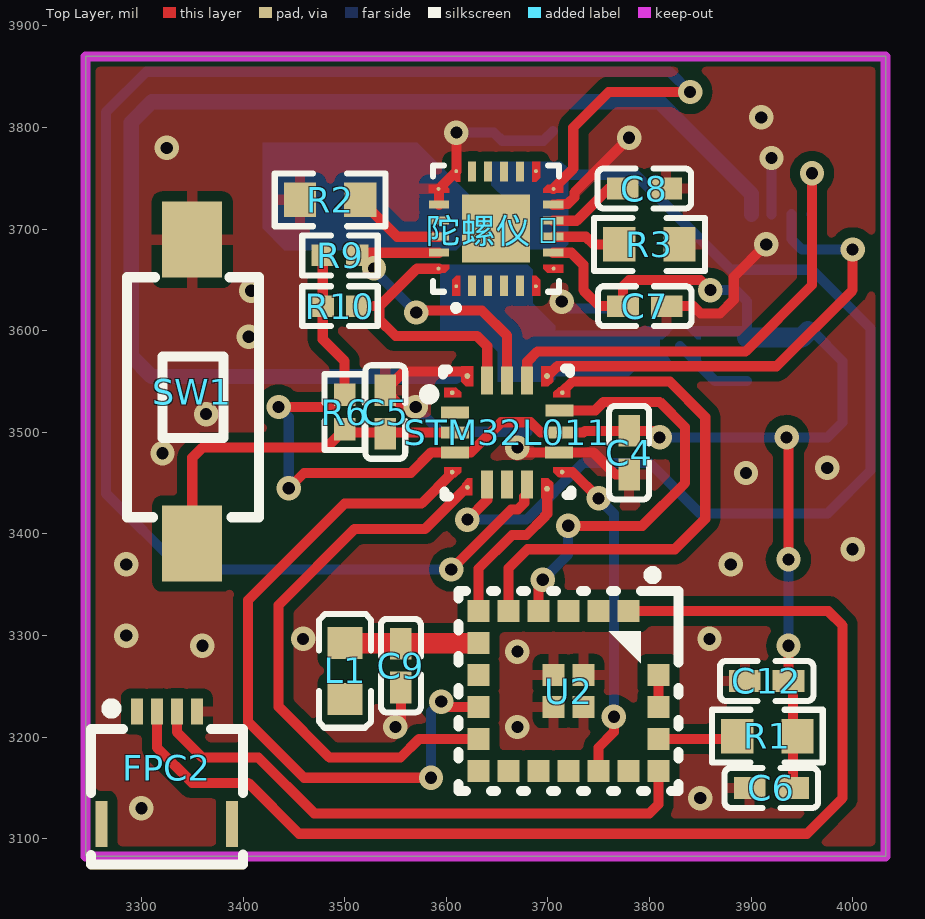
[diagram p0: Top Layer view]
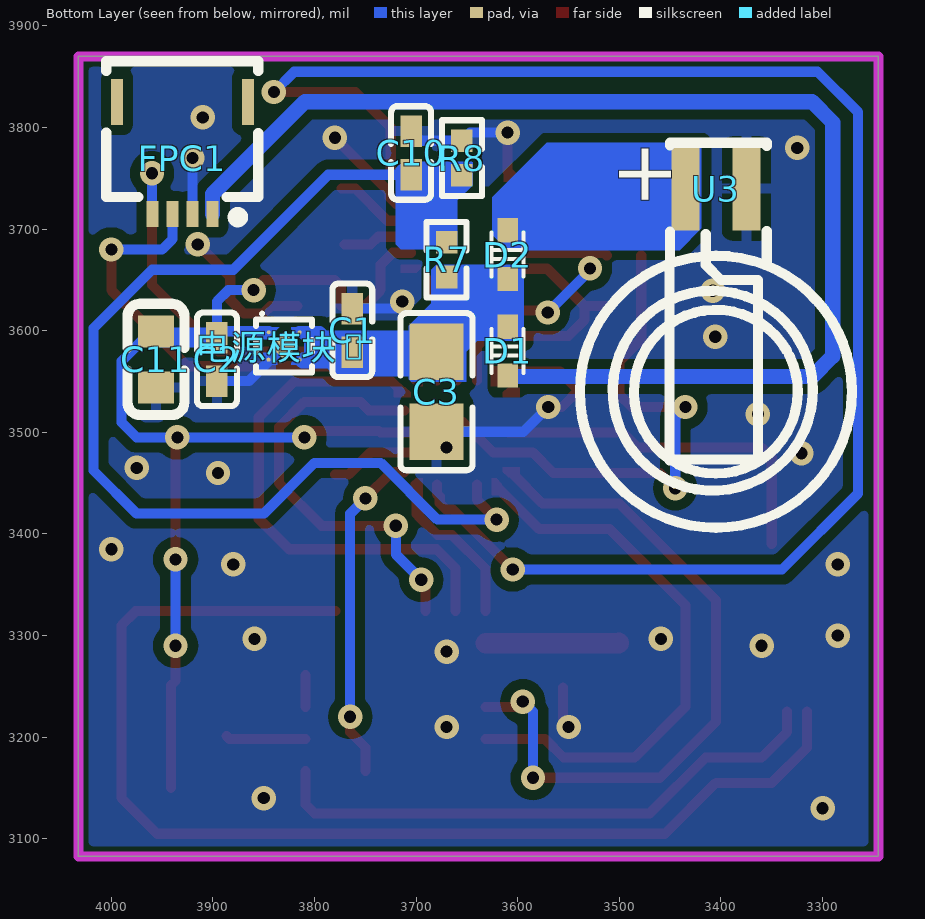
[diagram p1: Bottom Layer view, seen from below]
# Altium PCB MISC50958.pcbdoc
Units mil, origin at the board's own origin, x right, y up, seen from the top; angles counter-clockwise.
Board outline 787.4 x 787.4 mil, 2 copper layers (Top Layer, Bottom Layer), stack 62.206 mil thick; 31 components, 27 nets, 136 pads, 47 vias.

## Layer stack, top to bottom
Top Solder Mask Layer: solder mask 0.394, Dk 3.3
Top Layer: signal copper 1.379
Dielectric1: surface 59.449, FR4, Dk 4.5
Bottom Layer: signal copper 1.378
Bottom Solder Mask Layer: solder mask 0.394, Dk 3.3

## Board outline
3245,3870 3245,3082.6 4032.4,3082.6 4032.4,3870

## Design rules (kind name [scope] priority, off if disabled: settings)
BoardOutlineClearance copperThickness2oz_1 [All] p2 off: genericclearance=7.99 ignorepadtopadclearanceinfootprint=FALSE except(0: Arc-SplitContinuation Track-SplitContinuation SMDPad-SplitContinuation THPad-SplitContinuation Via-SplitContinuation Fill-SplitContinuation Region-SplitContinuation Poly-SplitContinuation Text-SplitContinuation Hole-SplitContinuation; 5.98: Arc-OutlineEdge Track-OutlineEdge SMDPad-OutlineEdge THPad-OutlineEdge Via-OutlineEdge Fill-OutlineEdge Region-OutlineEdge Text-OutlineEdge Hole-OutlineEdge SMDPad-CutoutEdge THPad-CutoutEdge Via-CutoutEdge Fill-CutoutEdge Region-CutoutEdge Text-CutoutEdge Hole-CutoutEdge; 10: Poly-OutlineEdge Poly-CutoutEdge; 11.81: Arc-CutoutEdge Track-CutoutEdge)
BoardOutlineClearance Plane_innerPlane_1 [All] p4 off: genericclearance=4.02 ignorepadtopadclearanceinfootprint=FALSE except(0: Arc-SplitContinuation Track-SplitContinuation SMDPad-SplitContinuation THPad-SplitContinuation Via-SplitContinuation Fill-SplitContinuation Region-SplitContinuation Poly-SplitContinuation Text-SplitContinuation Hole-SplitContinuation; 5.98: Arc-OutlineEdge Track-OutlineEdge SMDPad-OutlineEdge THPad-OutlineEdge Via-OutlineEdge Fill-OutlineEdge Region-OutlineEdge Text-OutlineEdge Hole-OutlineEdge SMDPad-CutoutEdge THPad-CutoutEdge Via-CutoutEdge Fill-CutoutEdge Region-CutoutEdge Text-CutoutEdge Hole-CutoutEdge; 10: Poly-OutlineEdge Poly-CutoutEdge; 11.81: Arc-CutoutEdge Track-CutoutEdge)
BoardOutlineClearance Copper_copperRegion_1 [All] p6 off: genericclearance=4.02 ignorepadtopadclearanceinfootprint=FALSE except(0: Arc-SplitContinuation Track-SplitContinuation SMDPad-SplitContinuation THPad-SplitContinuation Via-SplitContinuation Fill-SplitContinuation Region-SplitContinuation Poly-SplitContinuation Text-SplitContinuation Hole-SplitContinuation; 5.98: Arc-OutlineEdge Track-OutlineEdge SMDPad-OutlineEdge THPad-OutlineEdge Via-OutlineEdge Fill-OutlineEdge Region-OutlineEdge Text-OutlineEdge Hole-OutlineEdge SMDPad-CutoutEdge THPad-CutoutEdge Via-CutoutEdge Fill-CutoutEdge Region-CutoutEdge Text-CutoutEdge Hole-CutoutEdge; 10: Poly-OutlineEdge Poly-CutoutEdge; 11.81: Arc-CutoutEdge Track-CutoutEdge)
BoardOutlineClearance copperThickness1oz_1 [All] p8: genericclearance=4.02 ignorepadtopadclearanceinfootprint=FALSE except(0: Arc-SplitContinuation Track-SplitContinuation SMDPad-SplitContinuation THPad-SplitContinuation Via-SplitContinuation Fill-SplitContinuation Region-SplitContinuation Poly-SplitContinuation Text-SplitContinuation Hole-SplitContinuation; 5.98: Arc-OutlineEdge Track-OutlineEdge SMDPad-OutlineEdge THPad-OutlineEdge Via-OutlineEdge Fill-OutlineEdge Region-OutlineEdge Text-OutlineEdge Hole-OutlineEdge SMDPad-CutoutEdge THPad-CutoutEdge Via-CutoutEdge Fill-CutoutEdge Region-CutoutEdge Text-CutoutEdge Hole-CutoutEdge; 10: Poly-OutlineEdge Poly-CutoutEdge; 11.81: Arc-CutoutEdge Track-CutoutEdge)
Clearance copperThickness2oz [All] p1 off: gap=7.99 ignorepadtopadclearanceinfootprint=FALSE except(5.98: SMDPad-Track SMDPad-SMDPad THPad-Track SMDPad-THPad THPad-THPad Track-Via SMDPad-Via THPad-Via Via-Via Fill-Track Region-Track Fill-SMDPad Region-SMDPad Fill-THPad Region-THPad Fill-Via Region-Via Fill-Fill Fill-Region Region-Region Arc-Track Arc-SMDPad Arc-THPad Arc-Via Fill-Arc Region-Arc Arc-Arc Text-Track SMDPad-Text Text-THPad Text-Via Fill-Text Region-Text Arc-Text Text-Text Hole-Track Hole-SMDPad Hole-THPad Hole-Via Fill-Hole Region-Hole Hole-Arc Hole-Text; 10: Poly-Track Poly-SMDPad Poly-THPad Poly-Via Poly-Fill Poly-Region Poly-Poly Poly-Arc Poly-Text Poly-Hole)
Clearance Plane_innerPlane [All] p3 off: gap=4.02 ignorepadtopadclearanceinfootprint=FALSE except(5.98: SMDPad-Track SMDPad-SMDPad THPad-Track SMDPad-THPad THPad-THPad Track-Via SMDPad-Via THPad-Via Via-Via Fill-Track Region-Track Fill-SMDPad Region-SMDPad Fill-THPad Region-THPad Fill-Via Region-Via Fill-Fill Fill-Region Region-Region Arc-Track Arc-SMDPad Arc-THPad Arc-Via Fill-Arc Region-Arc Arc-Arc Text-Track SMDPad-Text Text-THPad Text-Via Fill-Text Region-Text Arc-Text Text-Text Hole-Track Hole-SMDPad Hole-THPad Hole-Via Fill-Hole Region-Hole Hole-Arc Hole-Text; 10: Poly-Track Poly-SMDPad Poly-THPad Poly-Via Poly-Fill Poly-Region Poly-Poly Poly-Arc Poly-Text Poly-Hole)
Clearance Copper_copperRegion [All] p5 off: gap=4.02 ignorepadtopadclearanceinfootprint=FALSE except(5.98: SMDPad-Track SMDPad-SMDPad THPad-Track SMDPad-THPad THPad-THPad Track-Via SMDPad-Via THPad-Via Via-Via Fill-Track Region-Track Fill-SMDPad Region-SMDPad Fill-THPad Region-THPad Fill-Via Region-Via Fill-Fill Fill-Region Region-Region Arc-Track Arc-SMDPad Arc-THPad Arc-Via Fill-Arc Region-Arc Arc-Arc Text-Track SMDPad-Text Text-THPad Text-Via Fill-Text Region-Text Arc-Text Text-Text Hole-Track Hole-SMDPad Hole-THPad Hole-Via Fill-Hole Region-Hole Hole-Arc Hole-Text; 10: Poly-Track Poly-SMDPad Poly-THPad Poly-Via Poly-Fill Poly-Region Poly-Poly Poly-Arc Poly-Text Poly-Hole)
Clearance copperThickness1oz [All] p7: gap=4.02 ignorepadtopadclearanceinfootprint=FALSE except(5.98: SMDPad-Track SMDPad-SMDPad THPad-Track SMDPad-THPad THPad-THPad Track-Via SMDPad-Via THPad-Via Via-Via Fill-Track Region-Track Fill-SMDPad Region-SMDPad Fill-THPad Region-THPad Fill-Via Region-Via Fill-Fill Fill-Region Region-Region Arc-Track Arc-SMDPad Arc-THPad Arc-Via Fill-Arc Region-Arc Arc-Arc Text-Track SMDPad-Text Text-THPad Text-Via Fill-Text Region-Text Arc-Text Text-Text Hole-Track Hole-SMDPad Hole-THPad Hole-Via Fill-Hole Region-Hole Hole-Arc Hole-Text; 10: Poly-Track Poly-SMDPad Poly-THPad Poly-Via Poly-Fill Poly-Region Poly-Poly Poly-Arc Poly-Text Poly-Hole)
DiffPairsRouting differentialPair [All] p1: maxlimit=6 minlimit=6 mostfreqgap=6 toplayer_minwidth=5 toplayer_prefwidth=10 toplayer_maxwidth=100 toplayer_mingap=6 toplayer_prefgap=6 toplayer_maxgap=6 bottomlayer_minwidth=5 bottomlayer_prefwidth=10 bottomlayer_maxwidth=100 bottomlayer_mingap=6 bottomlayer_prefgap=6 bottomlayer_maxgap=6 maxuncoupledlength=10
HoleToHoleClearance otherClearance [All] p1: gap=11.8 allowstackedmicrovias=TRUE
Length netLength [All] p1: minlimit=0 maxlimit=0
PasteMaskExpansion pasteMaskExpansion [All] p1: expansion=0
PlaneConnect innerPlane [All] p1: planeconnectstyle=Relief reliefexpansion=20 reliefentries=4 reliefconductorwidth=10 reliefairgap=10
PolygonConnect copperRegion [(InNet('GND'))] p1: connectstyle=Relief reliefconductorwidth=10 reliefentries=4 polygonreliefangle="90 Angle" airgapwidth=10 via.connectstyle=Relief via.reliefconductorwidth=10 via.reliefentries=4 via.polygonreliefangle="90 Angle" via.airgapwidth=10
RoutingVias viaSize [All] p1: holewidth=12.01 width=24.02 viastyle="Through Hole" minholewidth=11.81 minwidth=19.68 maxholewidth=248.03 maxwidth=393.7
SolderMaskExpansion solderMaskExpansion [IsVia] p1: expansion=-1000 istentingtop=TRUE
SolderMaskExpansion solderMaskExpansion [All] p2: expansion=2 istentingtop=FALSE
Width copperThickness2oz_2 [All] p1 off: maxlimit=100 minlimit=8 preferedwidth=10
Width copperThickness1oz_2 [All] p2: maxlimit=100 minlimit=5 preferedwidth=10

## Components (designator, comment, footprint, x,y, rotation, side; value= is the part's Value field where it differs from the comment)
C1 "1uF" C0402 3762.88,3600.39 r270 bottom
C2 "1uF" C0402 3896.09,3571.84 r90 bottom
C3 "10uF" C0805 3680,3540 r90 bottom
C4 "1uF" C0402 3780,3480 r90 top
C5 "100nF" C0402 3540,3520 r270 top
C6 "100nF" C0402 3920,3150 r0 top
C7 "100nF" C0402 3795.44,3624.22 r180 top
C8 "100nF" C0402 3795,3740 r0 top
C9 "100nF" C0402 3555.37,3270.32 r90 top
C10 "1uF" C0402 3705,3775 r270 bottom
C11 "100nF" C0603 3956.09,3571.84 r90 bottom
C12 "100nF" C0402 3915.37,3255.32 r0 top
D1 "1N4148G" SOD-723_L1.0-W0.6-P1.4-RD 3610,3580 r270 bottom
D2 "1N4148G" SOD-723_L1.0-W0.6-P1.4-RD 3610,3675 r90 bottom
FPC1 "HC-FPC-05-10-4RLTAG" FPC-SMD_4P-P0.50_HCTL_HC-FPC-05-10-4RLTAG 3930,3770 r180 bottom
FPC2 "HC-FPC-05-10-4RLTAG" FPC-SMD_4P-P0.50_HCTL_HC-FPC-05-10-4RLTAG 3325,3170 r180 top
L1 "10uH" L0603 3500.37,3265.32 r90 top
R1 "10K" R0603 3916.06,3201 r0 top
R2 "10K" R0603 3485.78,3728.88 r0 top
R3 "10K" R0603 3800,3685 r180 top
R6 "10kΩ" R0402 3500,3520 r270 top
R7 "20kΩ" R0402 3670,3670 r270 bottom
R8 "10kΩ" R0402 3655,3770 r270 bottom
R9 "4.7kΩ" R0402 3495.44,3674.22 r0 top
R10 "4.7kΩ" R0402 3495.44,3624.22 r0 top
STM32L011 "STM32L011F4U6TR" QFN-20_L3.0-W3.0-P0.50-BL 3660,3500 r180 top
SW1 "TS-1101-C-W" SW-SMD_L6.0-W3.3-LS8.0 3350,3540 r90 top
U2 "HJ-185IMH" LGA-24_L5.5-W5.0-P0.75-BL-EP 3720.37,3245.32 r180 top
U3 "MS621FE-FL11E" BAT-SMD_FL11E 3405,3740 r90 bottom
电源模块1 "1.8V转压" ZQFN-4L_L1.0-W1.0-P0.63-BL-EP 3830,3585 r270 bottom
陀螺仪1 "ICM-20948" QFN-24_L3.0-W3.0-P0.40-BL-EP 3649.05,3700.44 r0 top

## Footprints (in the part's own frame and the unit in brackets; to place one, negate y for a bottom-side part, rotate by r counter-clockwise, add the part's x,y. Pads: shape width x height; smd on the part's side, far side on the other; paste and mask are expansions set on the pad)
BAT-SMD_FL11E [mm]
  rect 2.1x0.7 smd paste+0 mask+0.05: 1(0,0.762) 2(0,-0.762)
  silkscreen extent -8.48,-3.4 1.14,3.4
C0402 [mm]
  rect 0.79x0.54 smd paste-100 mask+0.051: 1(-0.545,0) 2(0.545,0)
  silkscreen extent -1.17,-0.5 1.17,0.5
C0603 [mm]
  rect 0.8x0.9 smd: 1(-0.7,0) 2(0.7,0)
  silkscreen extent -1.39,-0.71 1.39,0.71
C0805 [mm]
  rect 1.41x1.35 smd paste-100 mask+0.051: 1(-1,0) 2(1,0)
  silkscreen extent -1.96,-0.9 1.96,0.9
FPC-SMD_4P-P0.50_HCTL_HC-FPC-05-10-4RLTAG [mm]
  rect 0.3x0.65 smd paste+0 mask+0.05: 1(0.75,-1.405) 2(0.25,-1.405) 3(-0.25,-1.405) 4(-0.75,-1.405)
  rect 0.3x1.15 smd paste+0 mask+0.05: 5(-1.635,1.405) 6(1.635,1.405)
  silkscreen extent -1.9,-1.6 1.89,2.42
L0603 [mm]
  rect 0.8x0.864 smd paste-100 mask+0.051: 1(-0.7,0) 2(0.7,0)
  silkscreen extent -1.42,-0.65 1.42,0.65
LGA-24_L5.5-W5.0-P0.75-BL-EP [mm]
  rect 0.55x0.55 smd paste+0 mask+0.05: 1(-1.5,-2) 2(-0.75,-2) 3(0,-2) 4(0.75,-2) 5(1.5,-2) 6(2.25,-2) 7(2.25,-1.2) 8(2.25,-0.4) 9(2.25,0.4) 10(2.25,1.2) 11(2.25,2) 12(1.5,2) 13(0.75,2) 14(0,2) 15(-0.75,2) 16(-1.5,2) 17(-2.25,2) 18(-2.25,1.2) 19(-2.25,0.4) 20(-2.25,-0.4) 21(-0.375,0.4) 22(0.375,0.4) 23(0.375,-0.4) 24(-0.375,-0.4)
  silkscreen extent -2.75,-3 2.75,2.5
QFN-20_L3.0-W3.0-P0.50-BL [mm]
  round 0.117 smd: 1(1.378,-0.99) 5(1.377,0.993) 6(0.994,1.377) 11(-1.373,0.992) 15(-1.378,-0.993)
  rect 0.7x0.3 smd paste+0 mask+0.05: 2(1.301,-0.5) 3(1.301,0) 4(1.301,0.5) 12(-1.299,0.5) 13(-1.299,0) 14(-1.312,-0.55)
  rect 0.3x0.7 smd paste+0 mask+0.05: 7(0.501,1.3) 8(0.001,1.3) 9(-0.499,1.3) 17(-0.499,-1.3) 18(0.001,-1.3) 19(0.501,-1.3)
  round 0.145 smd: 10(-0.994,1.41) 16(-0.994,-1.41) 20(0.996,-1.41)
  Top Layer region: 1.151,-1.65 0.851,-1.65 0.851,-1.15 1.031,-1.15 1.151,-1.26
  Top Layer region: -1.149,-1.65 -0.849,-1.65 -0.849,-1.15 -1.029,-1.15 -1.149,-1.26
  Top Layer region: -1.149,1.65 -0.849,1.65 -0.849,1.15 -1.029,1.15 -1.149,1.26
  Top Layer region: 1.574,1.124 1.574,0.878 1.497,0.876 1.15,0.876 1.15,0.999 1.289,1.125
  Top Layer region: 1.125,1.574 0.878,1.574 0.877,1.496 0.877,1.149 1,1.149 1.126,1.288
  Top Layer region: -1.575,-1.125 -1.575,-0.877 -1.151,-0.877 -1.151,-1 -1.29,-1.126
  Top Layer region: -1.571,1.123 -1.571,0.876 -1.493,0.875 -1.146,0.875 -1.146,0.998 -1.285,1.124
  Top Layer region: 1.575,-1.121 1.575,-0.875 1.498,-0.873 1.151,-0.873 1.151,-0.997 1.29,-1.123
  silkscreen extent -1.6,-1.6 2.08,1.6
QFN-24_L3.0-W3.0-P0.40-BL-EP [mm]
  round 0.097 smd: 1(-0.996,-1.439) 6(0.997,-1.439) 7(1.439,-0.997) 12(1.439,0.996) 13(0.997,1.439) 18(-0.997,1.439) 19(-1.439,0.997) 24(-1.439,-0.997)
  rect 0.2x0.505 smd paste-100 mask+0.051: 2(-0.6,-1.427) 3(-0.2,-1.427) 4(0.2,-1.427) 5(0.6,-1.427) 14(0.6,1.427) 15(0.2,1.427) 16(-0.2,1.427) 17(-0.6,1.427)
  rect 0.505x0.2 smd paste-100 mask+0.051: 8(1.427,-0.6) 9(1.427,-0.2) 10(1.427,0.2) 11(1.427,0.6) 20(-1.427,0.6) 21(-1.427,0.2) 22(-1.427,-0.2) 23(-1.427,-0.6)
  rect 1.7x1.7 smd paste-100 mask+0.051: 25(0,0)
  Top Layer region: -1.1,1.68 -0.9,1.68 -0.9,1.175 -1,1.174 -1.1,1.274
  Top Layer region: -1.68,-1.1 -1.274,-1.1 -1.174,-1 -1.175,-0.9 -1.68,-0.9
  Top Layer region: 1.68,-1.1 1.275,-1.1 1.175,-1 1.175,-0.9 1.68,-0.9
  Top Layer region: 1.68,1.1 1.274,1.1 1.174,1 1.175,0.9 1.68,0.9
  Top Layer region: 1.1,1.68 0.9,1.68 0.9,1.175 1,1.174 1.1,1.274
  Top Layer region: -1.1,-1.68 -0.9,-1.68 -0.9,-1.175 -1,-1.174 -1.1,-1.275
  Top Layer region: 1.1,-1.68 0.9,-1.68 0.9,-1.175 1,-1.175 1.1,-1.275
  Top Layer region: -1.68,1.1 -1.274,1.1 -1.174,1 -1.175,0.9 -1.68,0.9
  silkscreen extent -1.58,-2.05 1.58,1.58
R0402 [mm]
  rect 0.566x0.54 smd paste-100 mask+0.051: 1(-0.433,0) 2(0.433,0)
  silkscreen extent -0.94,-0.5 0.94,0.5
R0603 [mil]
  rect 31.75x34.02 smd paste-3937.01 mask+2: 1(-29.66,0) 2(29.66,0)
  silkscreen extent -55,-26 55,26
SOD-723_L1.0-W0.6-P1.4-RD [mil]
  rect 24x20 smd: 1(-24.05,0) 2(24.05,0)
  silkscreen extent -22,-16 22,16
SW-SMD_L6.0-W3.3-LS8.0 [mm]
  rect 1.9x1.5 smd: 1(-3.8,0) 2(3.8,0)
  silkscreen extent -3.14,-1.67 2.86,1.63
ZQFN-4L_L1.0-W1.0-P0.63-BL-EP [mm]
  round 0.099 smd: 1(-0.343,-0.385)
  round 0.101 smd: 2(0.341,-0.389)
  round 0.1 smd: 3(0.341,0.389) 4(-0.341,0.389)
  rect 0.5x0.5 smd rot 45: 5(0,0)
  Top Layer region: -0.163,-0.525 -0.463,-0.525 -0.463,-0.125 -0.163,-0.425
  Top Layer region: 0.163,0.525 0.463,0.525 0.463,0.175 0.413,0.175 0.163,0.425
  Top Layer region: -0.463,0.175 -0.463,0.525 -0.163,0.525 -0.163,0.475 -0.163,0.425 -0.413,0.175
  Top Layer region: 0.463,-0.175 0.463,-0.525 0.163,-0.525 0.163,-0.425 0.413,-0.175
  silkscreen extent -0.83,-0.7 0.66,0.7

## Via types
v1: diameter 24.02, hole 12, Top Layer to Bottom Layer, 47 vias

## Nets (pads, with @x,y where several pads share a name; then routed paths per layer and width w, separated by ;. In a path a pad name is that pad's centre, name@x,y a point inside that pad or via, vN(x,y) a via of type N, cw(c..) or ccw(c..) an arc to the next point about the centre after c; other vN are vias at no path point)
3.3V: D1.2 FPC1.1 | length 1235.2
  Bottom Layer w15: D1.2 3609.05,3555 3310,3555 3290,3575 3290,3805 3310.5,3825.5 3809.5,3825.5 3900.47,3734.53 FPC1.1
$1N2563: C8.1 陀螺仪1.10 | length 81.4
  Top Layer w10: 陀螺仪1.10 3728.31,3708.31 3760,3740 C8.1
$1N2566: U2.19 U2.20 | length 31.5
  Top Layer w10: U2.19 U2.20
$1N3256: R1.1 U2.18 | length 78.7
  Top Layer w10: U2.18 3883.47,3198.07 R1.1
$1N3260: R2.2 陀螺仪1.22 | length 92.4
  Top Layer w10: R2.2 3551.75,3692.57 陀螺仪1.22
$1N3265: C9.2 L1.2 U2.7 | length 131.6
  Top Layer w20: L1.2 3500.68,3292.55 U2.7
$1N3266: R3.2 陀螺仪1.9 | length 68.2
  Top Layer w10: 陀螺仪1.9 3737.43,3692.57 3745,3685 R3.2
$1N3268: D2.2 U3.1
BATADC: C10.2 R7.1 R8.2 STM32L011.7 | length 1015.9
  Top Layer w10: v1(3620.86,3414.14) 3640.29,3433.56 STM32L011.7
  Bottom Layer w10: v1(3620.86,3414.14) 3679.14,3414.14 3735,3470 3800,3470 3850,3420 3975,3420 4017.5,3462.5 4017.5,3602.5 3960,3660 3880,3660 3786.46,3753.54 C10.2
BLE_CLK: FPC2.2 U2.1 | length 1146.4
  Top Layer w10: FPC2.2 3315.16,3189.84 3350,3155 3405,3155 3455,3105 3955,3105 3990,3140 3990,3310 3975.95,3324.05 U2.1
BLE_SWD: FPC2.3 U2.17 | length 563.8
  Top Layer w10: FPC2.3 3334.84,3205.16 3360,3180 3415,3180 3470,3125 3800,3125 3808.95,3133.95 U2.17
BLUE-RESET: STM32L011.8
BLUE_RX: STM32L011.15 U2.5 | length 516.3
  Top Layer w10: U2.5 3661.31,3366.31 3680,3385 3825,3385 3855,3415 3855,3515 3820,3550 3724.26,3550 STM32L011.15@3713.67,3539.41
BLUE_TX: STM32L011.14 U2.4 | length 420.6
  Top Layer w10: U2.4 3690.84,3350.84 v1(3695,3355) ; STM32L011.14 3746.66,3521.66 3755,3530 3810,3530 3835,3505 3835,3450 3792.99,3407.99 v1(3720,3407.99)
  Bottom Layer w10: v1(3695,3355) 3720,3380 v1(3720,3407.99)
GND: C1.1 C2.1 C3.1 C4.1 C5.1 C6.1 C7.1 C8.2 C9.1 C10.1 C11.1 C12.1 FPC1.2 FPC2.4 R2.1 R3.1 R8.1 STM32L011.12 STM32L011.20 SW1.2 U2.21 U2.22 U2.23 U2.24 U3.2 电源模块1.2 电源模块1.5 陀螺仪1.11 陀螺仪1.18 陀螺仪1.19 陀螺仪1.20 | length 1030.5
  Top Layer w10: v1(3550,3210) 3555.37,3215.37 C9.1 ; v1(3570,3525) 3556.46,3525 C5.1 3558.54,3560 3615.72,3560 STM32L011.20@3620.61,3555.12 ; 陀螺仪1.20 3592.85,3739.81 3609.68,3756.64 3610,3756.96 v1(3610,3795) ; v1(3670,3485) 3674.68,3480.32 STM32L011.12 3744.68,3480.32 3766.46,3458.54 C4.1 ; 陀螺仪1.11 陀螺仪1.11@3709.32,3724.06 ; v1(3780,3790) 3726.18,3736.18 3726.18,3731.32 3719.74,3724.89 陀螺仪1.11@3714.89,3724.89 ; C7.1 3843.27,3624.22 3850.48,3617.01 3869.52,3617.01 3882.99,3630.48 3882.99,3652.99 v1(3915,3685) ; 陀螺仪1.11@3709.32,3724.06 3710.15,3724.89 陀螺仪1.11@3714.89,3724.89 ; 陀螺仪1.11@3709.32,3724.06 3714.06,3724.06 陀螺仪1.11@3714.89,3724.89
  Bottom Layer w10: v1(3570,3525) 3594.37,3500.63 C3.1 ; v1(3610,3795) 3647.04,3795 R8.1 3695.58,3787.04 C10.1 ; v1(3713.74,3628.74) 3720.64,3621.85 C1.1 ; 电源模块1.5 3864.62,3550.38 C2.1 ; FPC1.2 v1(3920.16,3770)
  other v1: 3300,3130 3850,3140 3670,3210 3670,3284.22 3360,3290 3459.1,3296.7 3859.1,3296.7 3285,3300 3285,3370 3880,3370 4000,3385 3895,3460 3975,3465.04 3320.7,3479.41 3363.62,3518 3405.59,3594.1 3408.14,3639.45 3325,3780 3910,3810
INT: STM32L011.9 陀螺仪1.12 | length 1662.3
  Top Layer w10: v1(3605,3365) 3664.06,3424.06 3670.42,3424.06 3676.86,3430.49 3676.86,3436.86 3679.66,3439.66 STM32L011.9 ; 陀螺仪1.12@3705.25,3739.81 3725,3759.56 3725,3800 3760,3835 v1(3840,3835)
  Bottom Layer w10: v1(3605,3365) 3340,3365 3265,3440 3265,3815 3305,3855 3820,3855 v1(3840,3835)
NRST: C5.2 R6.2 STM32L011.3 SW1.1 | length 356.2
  Top Layer w10: SW1.1 3350,3475 3360,3485 3482.04,3485 R6.2 3502.96,3500 STM32L011.3
P0.00: STM32L011.6 U2.10 | length 558.8
  Top Layer w10: STM32L011.6@3620.59,3446.38 3579.21,3405 3510,3405 3435,3330 3435,3230 3485,3180 3555,3180 3573.07,3198.07 U2.10
P0.01: STM32L011.5 U2.9 | length 694.4
  Top Layer w10: v1(3585,3160) 3460,3160 3405,3215 3405,3335 3500,3430 3575.77,3430 STM32L011.5@3606.37,3460.61 ; v1(3595,3235) 3600.43,3229.57 U2.9
  Bottom Layer w10: v1(3585,3160) 3585,3225 v1(3595,3235)
P0.18: STM32L011.11 U2.15 | length 329.5
  Top Layer w10: STM32L011.11@3712,3460.67 3724.33,3460.67 v1(3750,3435) ; U2.15 3749.9,3189.9 3765,3205 v1(3765,3220)
  Bottom Layer w10: v1(3750,3435) 3765,3420 v1(3765,3220)
SCL: R9.2 STM32L011.18 陀螺仪1.23 | length 286.6
  Top Layer w10: R9.2 3515.08,3676.82 陀螺仪1.23 ; v1(3570.44,3617.99) 3572.45,3620 3635,3620 3659.97,3595.03 STM32L011.18
  Bottom Layer w10: v1(3528.9,3661.34) 3528.9,3659.54 v1(3570.44,3617.99)
SDA: R10.2 STM32L011.19 陀螺仪1.24 | length 259.5
  Top Layer w10: R10.2 3534.22,3624.22 ; 陀螺仪1.24@3592.85,3661.07 3571.07,3661.07 3534.22,3624.22 ; STM32L011.19 3640.29,3584.71 3630,3595 3550,3595 3534.22,3610.78 3534.22,3624.22
STATUS: STM32L011.10 U2.6 | length 157.1
  Top Layer w10: U2.6 3631.79,3365.93 3664.87,3399.02 3679.02,3399.02 3697.01,3417.01 3697.01,3417.52 3699.35,3419.85 STM32L011.10@3699.35,3444.88
SWCLK: FPC1.4 STM32L011.17 | length 480.5
  Top Layer w10: STM32L011.17 3679.66,3569.66 3689.66,3579.66 3894.66,3579.66 3960,3645 v1(3960,3755)
  Bottom Layer w10: FPC1.4 3960,3715.16 v1(3960,3755)
SWDIO: FPC1.3 STM32L011.16 | length 464.7
  Top Layer w10: STM32L011.16@3699.35,3555.12 3709.35,3565.12 3925.12,3565.12 4000,3640 v1(4000,3680)
  Bottom Layer w10: FPC1.3 3939.84,3690.16 3950,3680 v1(4000,3680)
VIN: C1.2 C3.2 D1.1 D2.1 R7.2 电源模块1.3 电源模块1.4 | length 90.1
  Bottom Layer w10: 电源模块1.3@3815.04,3570.51 3812.46,3567.93 3787.07,3567.93 3780,3575 3780,3585 3794.5,3599.5 电源模块1.4@3815.03,3599.5
VOUT-1.8V: C2.2 C4.2 C6.2 C7.2 C11.2 C12.2 R1.2 R6.1 R9.1 R10.1 STM32L011.4 STM32L011.13 电源模块1.1 陀螺仪1.8 | length 1749.7
  Top Layer w10: v1(3435,3525) 3484.74,3525 3484.82,3525.08 3488.04,3525.08 R6.1 3500,3570 3478.4,3591.6 R10.1 R9.1 ; v1(3445,3445) 3460,3460 3565,3460 3585.32,3480.32 STM32L011.4 3624.34,3480.32 3654.02,3510 3682.83,3510 3692.83,3500 STM32L011.13 3735,3500 3736.46,3501.46 C4.2 3803.54,3501.46 v1(3810,3495) ; 陀螺仪1.8 3723.18,3676.82 3735,3665 3735,3640 3750.78,3624.22 C7.2 3773.98,3643.98 3780,3650 3850,3650 v1(3860,3640) ; v1(3935,3495) 3936.83,3493.17 v1(3936.83,3375) ; v1(3936.83,3290) C12.2 3941.46,3250.68 C6.2
  Bottom Layer w10: v1(3435,3525) 3445,3515 v1(3445,3445) ; v1(3810,3495) v1(3935,3495) 3975,3495 3990,3510 3990,3570 3960.6,3599.4 C11.2 ; 电源模块1.1@3844.96,3599.49 3889.9,3599.49 C2.2 3896.09,3628.91 3885,3640 v1(3860,3640) ; v1(3936.83,3290) v1(3936.83,3375)
  Bottom Layer w20: C2.2 3949.99,3593.3 C11.2
pads on no net: FPC1.5 FPC1.6 FPC2.1 FPC2.5 FPC2.6 L1.1 STM32L011.1 STM32L011.2 U2.2 U2.3 U2.8 U2.11 U2.12 U2.13 U2.14 U2.16 陀螺仪1.1 陀螺仪1.2 陀螺仪1.3 陀螺仪1.4 陀螺仪1.5 陀螺仪1.6 陀螺仪1.7 陀螺仪1.13 陀螺仪1.14 陀螺仪1.15 陀螺仪1.16 陀螺仪1.17 陀螺仪1.21 陀螺仪1.25

## Polygon pours and split planes (outlines as drawn)
GND on Top Layer (solid, remove dead copper, pour order 0): 3000,3975 3000,3000 4150,3000 4150,3975
GND on Bottom Layer (solid, remove dead copper, pour order 2): 3155,3945 3155,3010 4110,3010 4110,3945

## Keep-outs
Board Outline Layer:
  the board outline again, w10

## Other copper
Bottom Layer:
  region net VIN: 3679.99,3665.01 3685,3660 3685,3627.32 3707.17,3605.16 3707.17,3552.17 3705,3550 3650.58,3550 3650.58,3579.42 3640,3590 3594.25,3590 3594.25,3664.25 3595.01,3665.01
  region net $1N3268: 3419.33,3785 3571.36,3785 3625,3731.36 3625,3694.33 3610,3679.33 3440.67,3679.33 3419.33,3700.67
  region net BATADC: 3645.12,3766.58 3713.42,3766.58 3720,3760 3720,3685 3715,3680 3659.37,3680 3659.37,3728.4 3644.37,3743.4 3644.37,3765.83
  region net VIN: 3700,3600 3783.33,3600 3795.44,3587.89 3795.44,3570.82 3779.74,3555.12 3699.35,3555.12 3699.35,3599.35
  region net VIN: 3805,3600 3810,3595 3810,3570.39 3812.46,3567.93 3787.07,3567.93 3780.32,3574.68 3780.32,3600